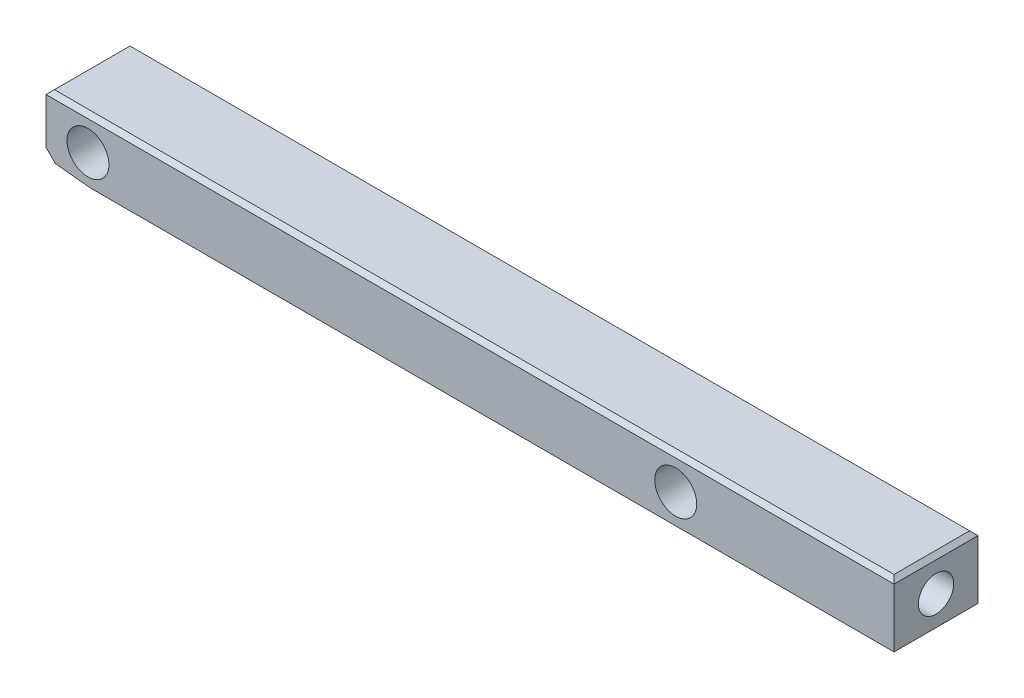
from build123d import *

# Parameters (mm, degrees)
BOSS_EXTRUDE1_DEPTH   = 5
SKETCH2_R             = 2.5
CUT_EXTRUDE1_DEPTH    = 52.635743434
CHAMFER1_SIZE         = 0.5
CHAMFER2_SIZE         = 1
CHAMFER2_SIZE2        = 1.123603797
M5_TAPPED_HOLE1_D     = 4.2
M5_TAPPED_HOLE1_DEPTH = 26
M5_TAPPED_HOLE1_TIP   = 1.2618073


with BuildPart() as part:
    # Sketch1 → Boss-Extrude1 (new, symmetric)
    with BuildSketch(Plane.XY):
        Polygon((-40.5, -4), (-50.5, -2.948957647), (-50.5, 4), (50.5, 4), (50.5, -4), align=None)
    extrude(amount=BOSS_EXTRUDE1_DEPTH, both=True)

    # Sketch2 → Cut-Extrude1 (cut, through all)
    with BuildSketch(Plane.XY.offset(5)):
        with Locations((-45.5, 0)):
            Circle(SKETCH2_R)
        with Locations((24.5, 0)):
            Circle(SKETCH2_R)
    extrude(amount=-CUT_EXTRUDE1_DEPTH, mode=Mode.SUBTRACT)

    # Chamfer1
    chamfer1_edges = [part.edges().sort_by_distance(p)[0] for p in [
        (5, -4, 5),
        (5, -4, -5),
        (0, 4, -5),
        (0, 4, 5),
        (50.5, -4, 0),
        (-50.5, 4, 0),
        (50.5, 4, 0),
    ]]
    chamfer(chamfer1_edges, length=CHAMFER1_SIZE)

    # Chamfer2
    chamfer2_edges = [part.edges().sort_by_distance(p)[0] for p in [
        (-50.5, -2.948957647, 0),
    ]]
    chamfer2_side = [part.faces().sort_by_distance(p)[0] for p in [
        (-50.5, 0.275521176, 0),
    ]]
    chamfer(chamfer2_edges, length=CHAMFER2_SIZE, length2=CHAMFER2_SIZE2, reference=chamfer2_side[0])

    # M5 Tapped Hole1
    with Locations(Plane(origin=(50.5, 0, 0), x_dir=(0, 0, -1), z_dir=(1, 0, 0))):
        with Locations((0, 0)):
            Hole(M5_TAPPED_HOLE1_D / 2, depth=M5_TAPPED_HOLE1_DEPTH)
            with Locations((0, 0, -(M5_TAPPED_HOLE1_DEPTH + M5_TAPPED_HOLE1_TIP / 2))):  # 118° drill point
                Cone(0, M5_TAPPED_HOLE1_D / 2, M5_TAPPED_HOLE1_TIP, mode=Mode.SUBTRACT)


solid = part.part
